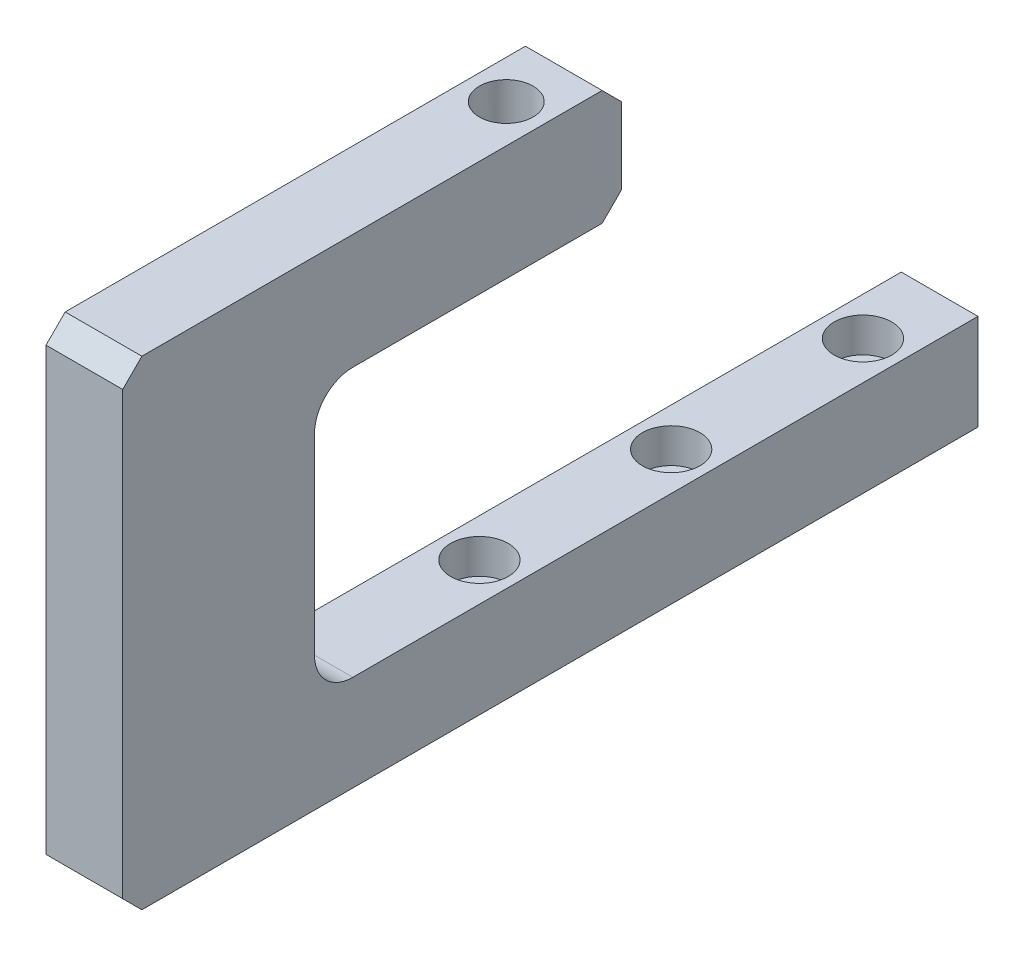
from build123d import *

# Parameters (mm, degrees)
SKETCH_1_W                = 20
SKETCH_1_H                = 25
EXTRUDE_1_DEPTH           = 223
HOLE_WIZARD_1_D           = 9
HOLE_WIZARD_1_CBORE_D     = 15
HOLE_WIZARD_1_CBORE_DEPTH = 9
PATTERN_LINEAR_1_COUNT    = 3
PATTERN_LINEAR_1_PITCH    = 50
SKETCH_6_W                = 20
SKETCH_6_H                = 50
EXTRUDE_3_DEPTH           = 70
SKETCH_7_W                = 20
SKETCH_7_H                = 130
EXTRUDE_4_DEPTH           = 30
HOLE_WIZARD_M16_1_D       = 14
HOLE_WIZARD_M16_1_DEPTH   = 38
HOLE_WIZARD_M16_1_TIP     = 4.206024333
CHAMFER_1_SIZE            = 5
FILLET_1_R                = 10
CHAMFER_2_SIZE            = 5


with BuildPart() as part:
    # 草图1 → 凸台-拉伸1 (new body)
    with BuildSketch(Plane.XY):
        Rectangle(SKETCH_1_W, SKETCH_1_H)
    extrude(amount=EXTRUDE_1_DEPTH)

    # 打孔尺寸(%根据)内六角圆柱头螺钉的类型1 (through all)
    with Locations(Plane(origin=(0, 12.5, 0), x_dir=(1, 0, 0), z_dir=(0, 1, 0))):
        with Locations((0, -20)):
            hole_wizard_1 = CounterBoreHole(HOLE_WIZARD_1_D / 2, HOLE_WIZARD_1_CBORE_D / 2, HOLE_WIZARD_1_CBORE_DEPTH)

    # 阵列(线性)1: 打孔尺寸(%根据)内六角圆柱头螺钉的类型1 ×3
    with Locations(*[(0, 0, i * PATTERN_LINEAR_1_PITCH) for i in range(1, PATTERN_LINEAR_1_COUNT)]):
        add(hole_wizard_1, mode=Mode.SUBTRACT)

    # 草图6 → 凸台-拉伸3 (add)
    with BuildSketch(Plane(origin=(0, 12.5, 0), x_dir=(1, 0, 0), z_dir=(0, 1, 0))):
        with Locations((0, -198)):
            Rectangle(SKETCH_6_W, SKETCH_6_H)
    extrude(amount=EXTRUDE_3_DEPTH)

    # 草图7 → 凸台-拉伸4 (add)
    with BuildSketch(Plane(origin=(0, 82.5, 0), x_dir=(1, 0, 0), z_dir=(0, 1, 0))):
        with Locations((0, -158)):
            Rectangle(SKETCH_7_W, SKETCH_7_H)
    extrude(amount=EXTRUDE_4_DEPTH)

    # M16 螺纹孔1
    with Locations(Plane(origin=(0, 112.5, 0), x_dir=(1, 0, 0), z_dir=(0, 1, 0))):
        with Locations((0, -113)):
            Hole(HOLE_WIZARD_M16_1_D / 2, depth=HOLE_WIZARD_M16_1_DEPTH)
            with Locations((0, 0, -(HOLE_WIZARD_M16_1_DEPTH + HOLE_WIZARD_M16_1_TIP / 2))):  # 118° drill point
                Cone(0, HOLE_WIZARD_M16_1_D / 2, HOLE_WIZARD_M16_1_TIP, mode=Mode.SUBTRACT)

    # 倒角1
    chamfer_1_edges = [part.edges().sort_by_distance(p)[0] for p in [
        (0, 82.5, 93),
        (0, 112.5, 93),
    ]]
    chamfer(chamfer_1_edges, length=CHAMFER_1_SIZE)

    # 圆角1
    fillet_1_edges = [part.edges().sort_by_distance(p)[0] for p in [
        (0, 12.5, 173),
        (0, 82.5, 173),
    ]]
    fillet(fillet_1_edges, radius=FILLET_1_R)

    # 倒角2
    chamfer_2_edges = [part.edges().sort_by_distance(p)[0] for p in [
        (0, -12.5, 223),
        (0, 112.5, 223),
    ]]
    chamfer(chamfer_2_edges, length=CHAMFER_2_SIZE)


solid = part.part
